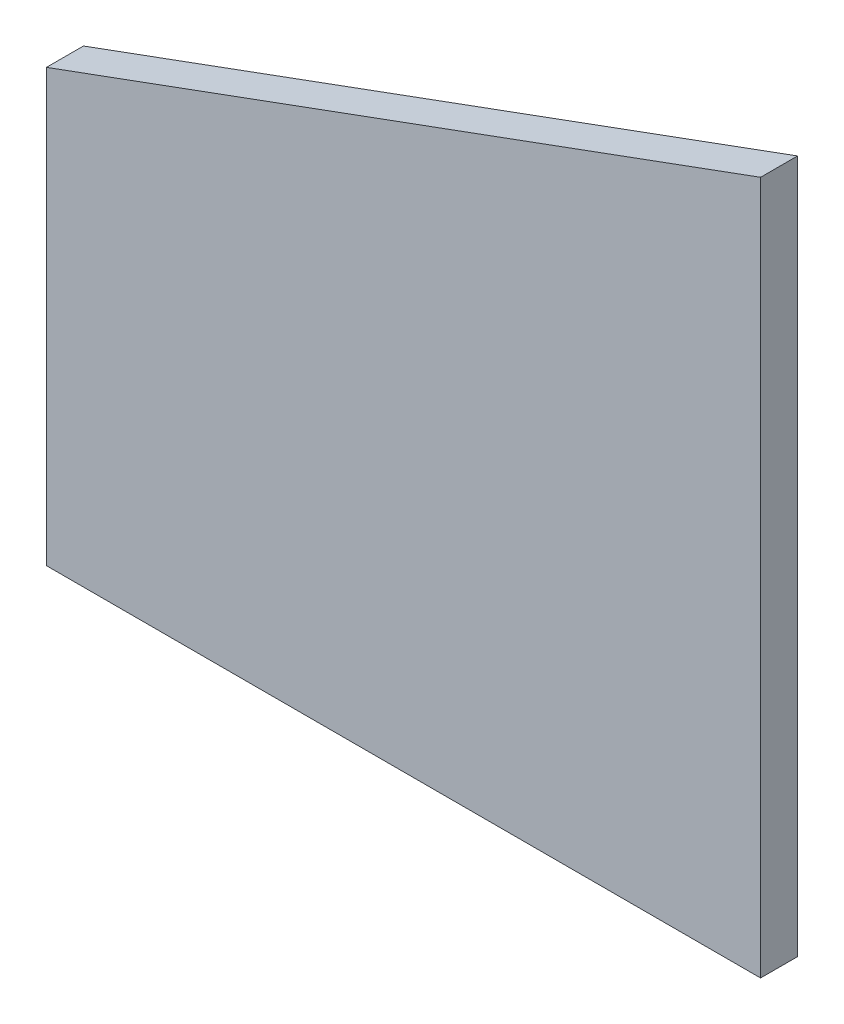
from build123d import *

# Parameters (mm, degrees)
EXTRUDE_1_DEPTH = 8


with BuildPart() as part:
    # 草图1 → 凸台-拉伸1 (new body)
    with BuildSketch(Plane.XY):
        Polygon((184.477803528, 193), (184.477803528, 286.35815759), (338.955555556, 343), (338.955555556, 193), align=None)
    extrude(amount=EXTRUDE_1_DEPTH)


solid = part.part
